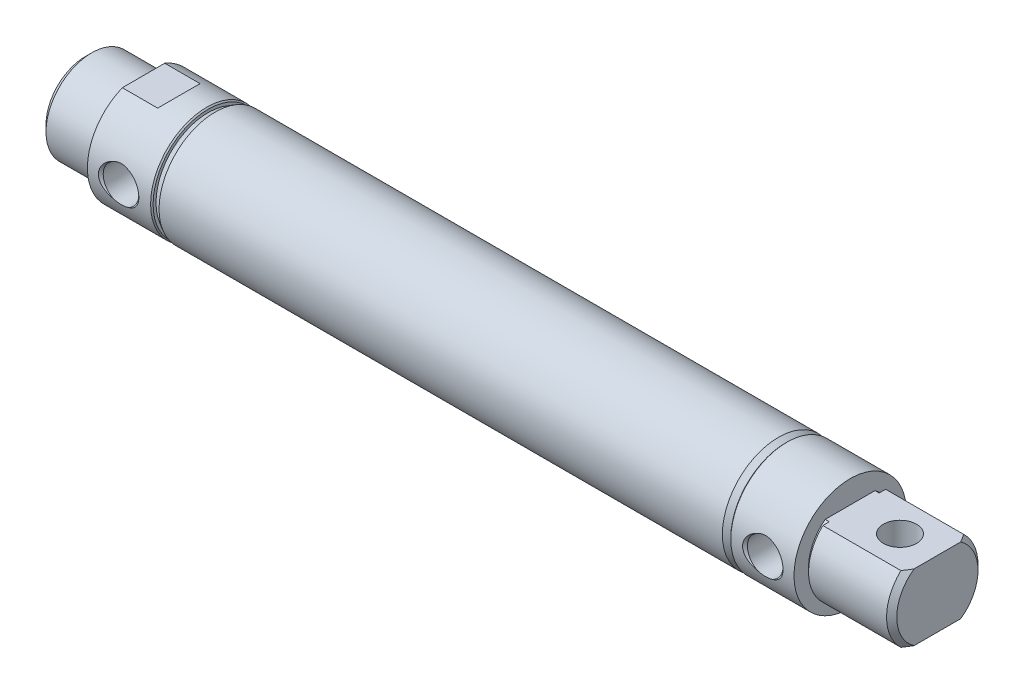
from build123d import *

# Parameters (mm, degrees)
CUT_EXTRUDE_1_DEPTH      = 13.5
CUT_EXTRUDE_1_DEPTH_BACK = 13.5
CUT_EXTRUDE_2_DEPTH      = 13.5
CUT_EXTRUDE_2_DEPTH_BACK = 13.5
CUT_EXTRUDE_3_DEPTH      = 13.5
CUT_EXTRUDE_3_DEPTH_BACK = 13.5
CUT_EXTRUDE_4_DEPTH      = 8
CUT_EXTRUDE_4_DEPTH_BACK = 8
SKETCH_5_R               = 4
SCALE_1_SCALE            = 0.5


with BuildPart() as part:
    # 草图1 → 旋转1 (revolve)
    with BuildSketch(Plane.XY, mode=Mode.PRIVATE) as revolve_1_sk:
        Polygon((154.5, 0), (154.5, 10), (15.5, 10), (15.5, 4), (-14, 4), (-14, 9.4665), (-12.4665, 11), (0, 11), (0, 13.5), (15.2, 13.5), (15.5, 13.2), (15.5, 12.5), (17.232050808, 13.5), (152.767949192, 13.5), (154.5, 12.5), (154.5, 13.2), (154.8, 13.5), (170, 13.5), (170, 10), (171, 10), (171, 11), (189.773, 11), (191, 9.773), (191, 0), align=None)
    revolve(revolve_1_sk.sketch.rotate(Axis((191, 0, 0), (-1, 0, 0)), 270), axis=Axis((191, 0, 0), (-1, 0, 0)))

    # 草图2 → 切除-拉伸1 (cut, two sides: drawn at the far end of the back side and taken through both)
    with BuildSketch(Plane.XY.offset(-CUT_EXTRUDE_1_DEPTH_BACK)):
        Polygon((0, 13.5), (0, 12.5), (8.5, 12.5), (9.5, 13.5), align=None)
    extrude(amount=CUT_EXTRUDE_1_DEPTH + CUT_EXTRUDE_1_DEPTH_BACK, mode=Mode.SUBTRACT)

    # 草图3 → 切除-拉伸2 (cut, two sides: drawn at the far end of the back side and taken through both)
    with BuildSketch(Plane.XY.offset(-CUT_EXTRUDE_2_DEPTH_BACK)):
        Polygon((0, -13.5), (9.5, -13.5), (8.5, -12.5), (0, -12.5), align=None)
    extrude(amount=CUT_EXTRUDE_2_DEPTH + CUT_EXTRUDE_2_DEPTH_BACK, mode=Mode.SUBTRACT)

    # 草图4 → 切除-拉伸3 (cut, two sides: drawn at the far end of the back side and taken through both)
    with BuildSketch(Plane.XY.offset(-CUT_EXTRUDE_3_DEPTH_BACK)):
        Polygon((170, 23), (170, 8), (192, 8), (192, -8), (170, -8), (170, -23), (197, -23), (197, 23), align=None)
    extrude(amount=CUT_EXTRUDE_3_DEPTH + CUT_EXTRUDE_3_DEPTH_BACK, mode=Mode.SUBTRACT)

    # 草图5 → 切除-拉伸4 (cut, two sides: drawn at the far end of the back side and taken through both)
    with BuildSketch(Plane(origin=(0, 0, 0), x_dir=(1, 0, 0), z_dir=(0, 1, 0)).offset(-CUT_EXTRUDE_4_DEPTH_BACK)):
        with Locations(Location((182, 0, 0), (0, 0, 270))):
            Circle(SKETCH_5_R)
    extrude(amount=CUT_EXTRUDE_4_DEPTH + CUT_EXTRUDE_4_DEPTH_BACK, mode=Mode.SUBTRACT)

    # 草图6 → 切除-旋转1 (revolve, cut)
    with BuildSketch(Plane(origin=(0, 0, 0), x_dir=(1, 0, 0), z_dir=(0, 1, 0)), mode=Mode.PRIVATE) as cut_revolve_1_sk:
        Polygon((7.5, -5), (11.783, -5), (11.783, -12.919), (12.364, -13.5), (7.5, -13.5), align=None)
    revolve(cut_revolve_1_sk.sketch.rotate(Axis((7.5, 0, 13.5), (0, 0, -1)), 180), axis=Axis((7.5, 0, 13.5), (0, 0, -1)), mode=Mode.SUBTRACT)

    # 草图7 → 切除-旋转2 (revolve, cut)
    with BuildSketch(Plane(origin=(0, 0, 0), x_dir=(1, 0, 0), z_dir=(0, 1, 0)), mode=Mode.PRIVATE) as cut_revolve_2_sk:
        Polygon((162.5, -4), (166.783, -4), (166.783, -12.919), (167.364, -13.5), (162.5, -13.5), align=None)
    revolve(cut_revolve_2_sk.sketch.rotate(Axis((162.5, 0, 13.5), (0, 0, -1)), 180), axis=Axis((162.5, 0, 13.5), (0, 0, -1)), mode=Mode.SUBTRACT)


with BuildPart() as part_1:
    # 缩放比例1: scaled about (88.257573556, -1e-09, -0.146875551)
    add(part.part.scale(SCALE_1_SCALE).moved(Location((44.128786778, -1e-09, -0.073437775))))


solid = part_1.part
